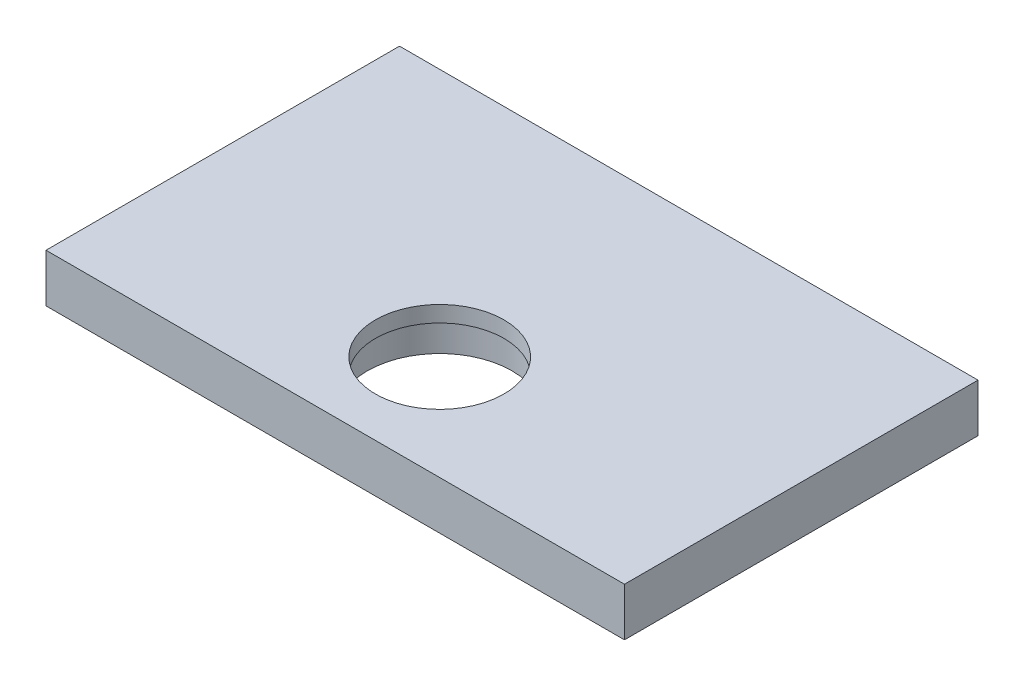
from build123d import *

# Parameters (mm, degrees)
SKETCH_1_W          = 360
SKETCH_1_H          = 220
EXTRUDE_1_DEPTH     = 30
SKETCH_2_R          = 40
CUT_EXTRUDE_1_DEPTH = 214.072757527
SKETCH_4_R          = 45
CUT_EXTRUDE_3_DEPTH = 20


with BuildPart() as part:
    # 草图1 → 凸台-拉伸1 (new body)
    with BuildSketch(Plane(origin=(0, 0, 0), x_dir=(1, 0, 0), z_dir=(0, 1, 0))):
        Rectangle(SKETCH_1_W, SKETCH_1_H)
    extrude(amount=EXTRUDE_1_DEPTH)

    # 草图2 → 切除-拉伸1 (cut, through all)
    with BuildSketch(Plane.XZ):
        with Locations(Location((0, 45, 0), (0, 0, 270))):
            Circle(SKETCH_2_R)
    extrude(amount=-CUT_EXTRUDE_1_DEPTH, mode=Mode.SUBTRACT)

    # 草图4 → 切除-拉伸3 (cut)
    with BuildSketch(Plane.XZ):
        with Locations(Location((0, 45, 0), (0, 0, 270))):
            Circle(SKETCH_4_R)
    extrude(amount=-CUT_EXTRUDE_3_DEPTH, mode=Mode.SUBTRACT)


solid = part.part
